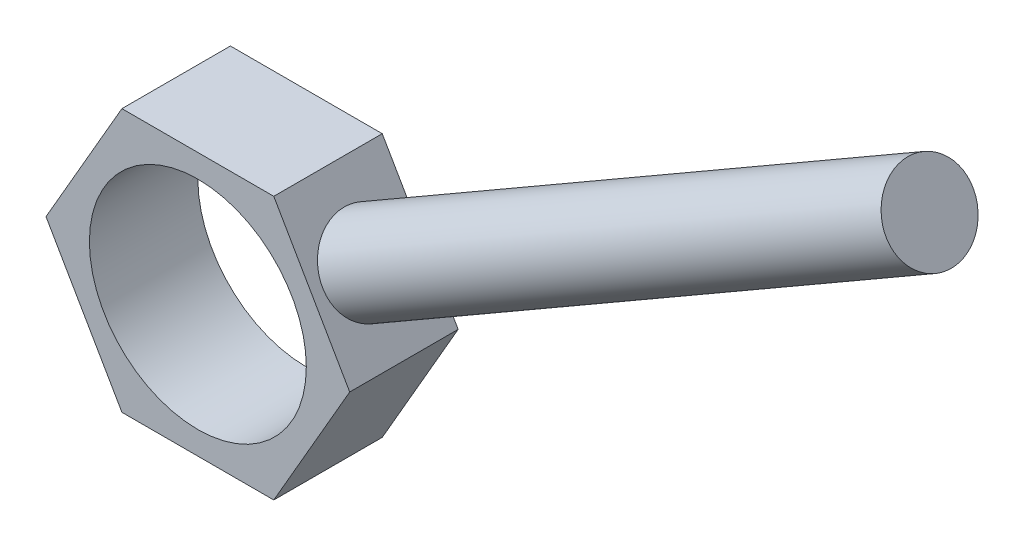
from build123d import *

# Parameters (mm, degrees)
SKETCH1_R           = 5
BOSS_EXTRUDE1_DEPTH = 5
SKETCH2_R           = 2
BOSS_EXTRUDE2_DEPTH = 30


with BuildPart() as part:
    # Sketch1 → Boss-Extrude1 (new body)
    with BuildSketch(Plane.XY):
        Polygon((-3.5, 6.062177826), (-7, 0), (-3.5, -6.062177826), (3.5, -6.062177826), (7, 0), (3.5, 6.062177826), align=None)
        Circle(SKETCH1_R, mode=Mode.SUBTRACT)
    extrude(amount=BOSS_EXTRUDE1_DEPTH)

    # Sketch2 → Boss-Extrude2 (add)
    with BuildSketch(Plane(origin=(5.25, 3.031088913, 0), x_dir=(0, 0, -1), z_dir=(0.8660254037844387, 0.49999999999999983, 0))):
        with Locations(Location((-2.5, 0, 0), (0, 0, 90))):
            Circle(SKETCH2_R)
    extrude(amount=BOSS_EXTRUDE2_DEPTH)


solid = part.part
